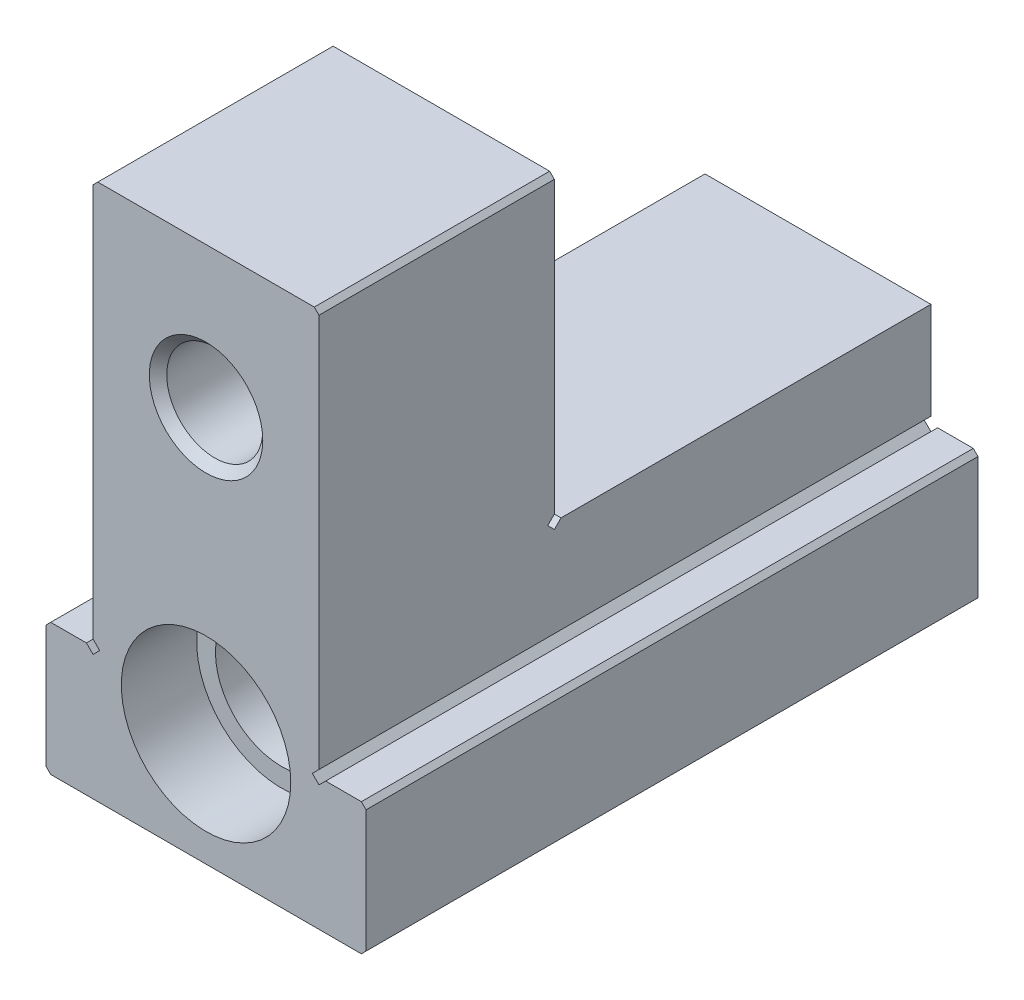
from build123d import *

# Parameters (mm, degrees)
BOSS_EXTRUDE1_DEPTH          = 65
CUT_EXTRUDE1_DEPTH           = 92.186621826
CUT_EXTRUDE1_DEPTH_BACK      = 92.186621826
SKETCH3_R                    = 9
CUT_EXTRUDE2_DEPTH           = 8
CUT_EXTRUDE3_START           = -8
SKETCH4_R                    = 9
CUT_EXTRUDE3_DEPTH           = 8
M16_TAPPED_HOLE1_D           = 14
M16_TAPPED_HOLE1_CSINK_D     = 16.05
M16_TAPPED_HOLE1_CSINK_ANGLE = 90
M12_TAPPED_HOLE1_D           = 10.2
M12_TAPPED_HOLE1_CSINK_D     = 12.05
M12_TAPPED_HOLE1_CSINK_ANGLE = 90


with BuildPart() as part:
    # Sketch1 → Boss-Extrude1 (new body)
    with BuildSketch(Plane.XY):
        Polygon((16.5, 0), (-16.5, 0), (-17, 0.5), (-17, 13.5), (-16.5, 14), (-12.707106781, 14), (-12, 13.292893219), (-11.292893219, 14), (-12, 14.707106781), (-12, 56.5), (-11.5, 57), (11.5, 57), (12, 56.5), (12, 14.707106781), (11.292893219, 14), (12, 13.292893219), (12.707106781, 14), (16.5, 14), (17, 13.5), (17, 0.5), align=None)
    extrude(amount=BOSS_EXTRUDE1_DEPTH)

    # Sketch2 → Cut-Extrude1 (cut, two sides: drawn at the far end of the back side and taken through both)
    with BuildSketch(Plane(origin=(12, 0, 0), x_dir=(0, 0, -1), z_dir=(1, 0, 0)).offset(-CUT_EXTRUDE1_DEPTH_BACK)):
        Polygon((-40, 79.715196203), (7.535961079, 79.715196203), (7.535961079, 25), (-39.292893219, 25), (-40, 24.292893219), (-40.707106781, 25), (-40, 25.707106781), align=None)
    extrude(amount=CUT_EXTRUDE1_DEPTH + CUT_EXTRUDE1_DEPTH_BACK, mode=Mode.SUBTRACT)

    # Sketch3 → Cut-Extrude2 (cut)
    with BuildSketch(Plane.XY.offset(65)):
        with Locations((0, 12)):
            Circle(SKETCH3_R)
    extrude(amount=-CUT_EXTRUDE2_DEPTH, mode=Mode.SUBTRACT)

    # Sketch4 → Cut-Extrude3 (cut)
    with BuildSketch(Plane(origin=(0, 0, 0), x_dir=(-1, 0, 0), z_dir=(0, 0, -1)).offset(CUT_EXTRUDE3_START)):
        with Locations(Location((0, 12, 0), (0, 0, 180))):
            Circle(SKETCH4_R)
    extrude(amount=CUT_EXTRUDE3_DEPTH, mode=Mode.SUBTRACT)

    # M16 Tapped Hole1 (through all)
    with Locations(Plane(origin=(0, 12, 8), x_dir=(-1, 0, 0), z_dir=(0, 0, -1))):
        with Locations((0, 0)):
            CounterSinkHole(M16_TAPPED_HOLE1_D / 2, M16_TAPPED_HOLE1_CSINK_D / 2, counter_sink_angle=M16_TAPPED_HOLE1_CSINK_ANGLE)

    # M12 Tapped Hole1 (through all)
    with Locations(Plane(origin=(0, 42, 65), x_dir=(1, 0, 0), z_dir=(0, 0, 1))):
        with Locations((0, 0)):
            CounterSinkHole(M12_TAPPED_HOLE1_D / 2, M12_TAPPED_HOLE1_CSINK_D / 2, counter_sink_angle=M12_TAPPED_HOLE1_CSINK_ANGLE)


solid = part.part
